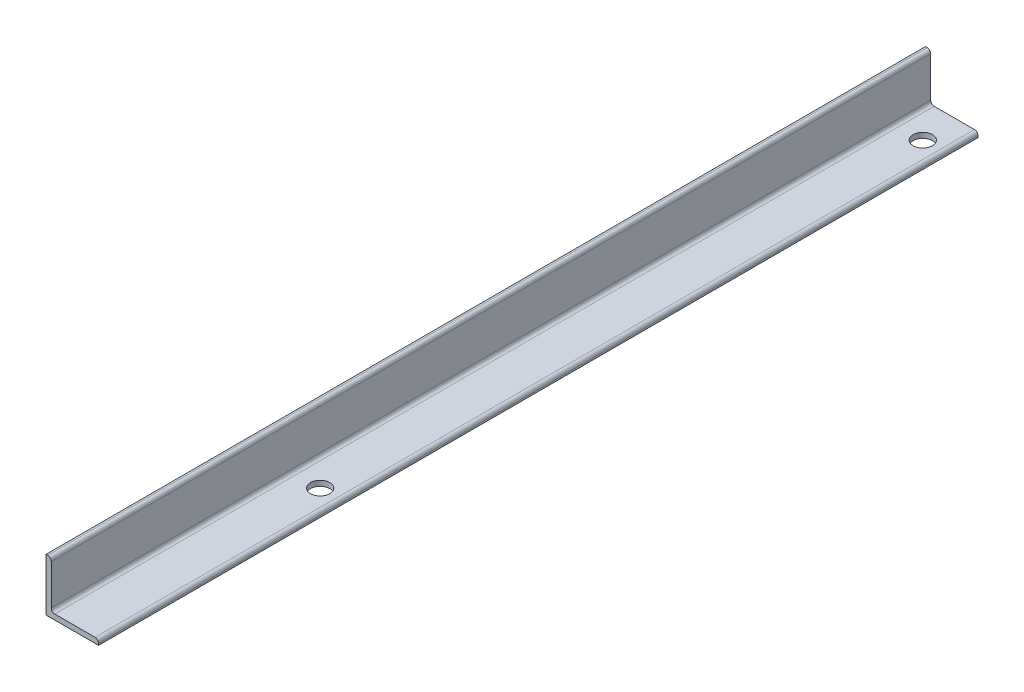
from build123d import *

# Parameters (mm, degrees)
BOSS_EXTRUDE1_DEPTH = 502
SKETCH2_R           = 5.5
CUT_EXTRUDE1_DEPTH  = 3
LPATTERN1_COUNT     = 2
LPATTERN1_PITCH     = 344


with BuildPart() as part:
    # Sketch1 → Boss-Extrude1 (new body)
    with BuildSketch(Plane.XY):
        with BuildLine():
            Line((0, 0), (30, 0))
            Line((30, 0), (30, 1))
            ThreePointArc((30, 1), (29.414213562, 2.414213562), (28, 3))
            Line((28, 3), (5, 3))
            ThreePointArc((5, 3), (3.585786438, 3.585786438), (3, 5))
            Line((3, 5), (3, 28))
            ThreePointArc((3, 28), (2.414213562, 29.414213562), (1, 30))
            Line((1, 30), (0, 30))
            Line((0, 30), (0, 0))
        make_face()
    extrude(amount=BOSS_EXTRUDE1_DEPTH)

    # Sketch2 → Cut-Extrude1 (cut)
    with BuildSketch(Plane.XZ):
        with Locations(Location((18.5, 20, 0), (0, 0, 270))):
            Circle(SKETCH2_R)
    cut_extrude1 = extrude(amount=-CUT_EXTRUDE1_DEPTH, mode=Mode.SUBTRACT)

    # LPattern1: Cut-Extrude1 ×2
    with Locations(*[(0, 0, i * LPATTERN1_PITCH) for i in range(1, LPATTERN1_COUNT)]):
        add(cut_extrude1, mode=Mode.SUBTRACT)


solid = part.part
